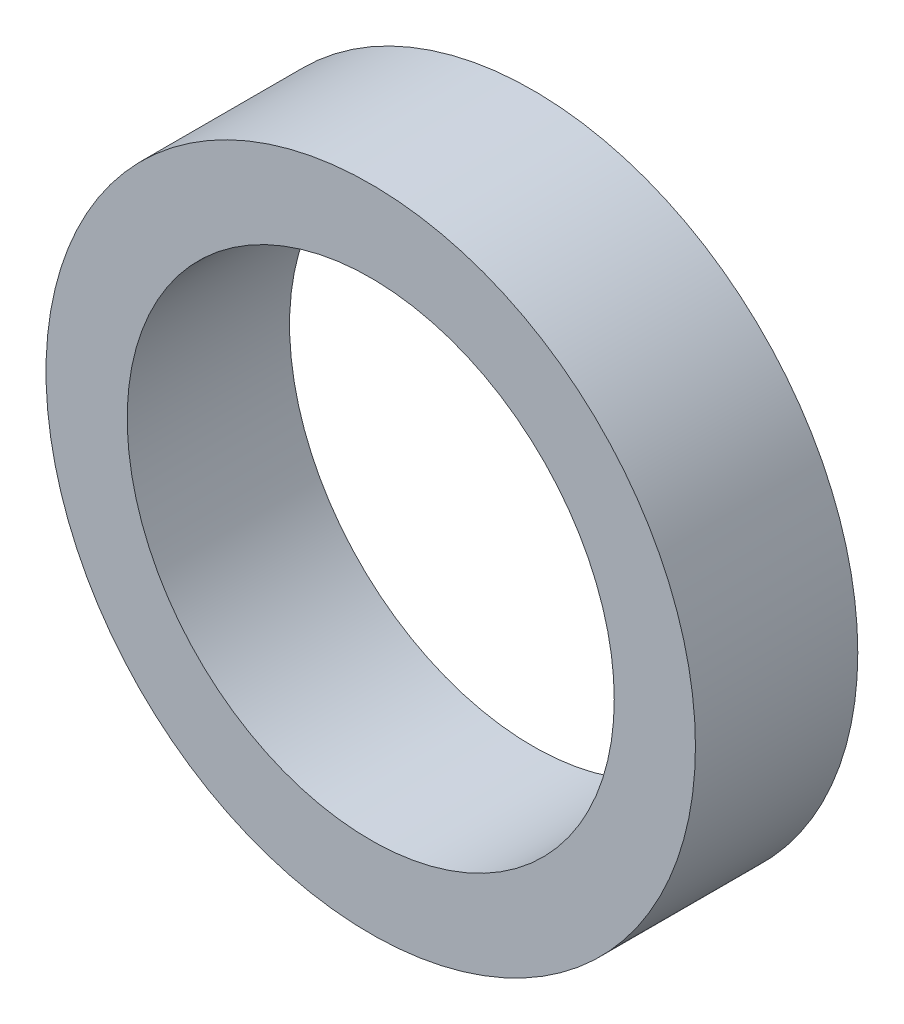
SolidWorks part; units mm, degrees
ref_plane "Front Plane" through (0, 0, 0) normal (0, 0, 1) x (1, 0, 0)
ref_plane "Top Plane" through (0, 0, 0) normal (0, 1, 0) x (1, 0, 0)
ref_plane "Right Plane" through (0, 0, 0) normal (1, 0, 0) x (0, 0, -1)
sketch "Sketch1" plane through (0, 0, 0) normal (0, 0, 1) x (1, 0, 0)
  circle A0 centre (0, 0) radius 4
  circle A1 centre (0, 0) radius 3
  dimension "D1" = 6
  dimension "D2" = 8
extrude "Boss-Extrude1" add sketch "Sketch1" along normal blind 2
